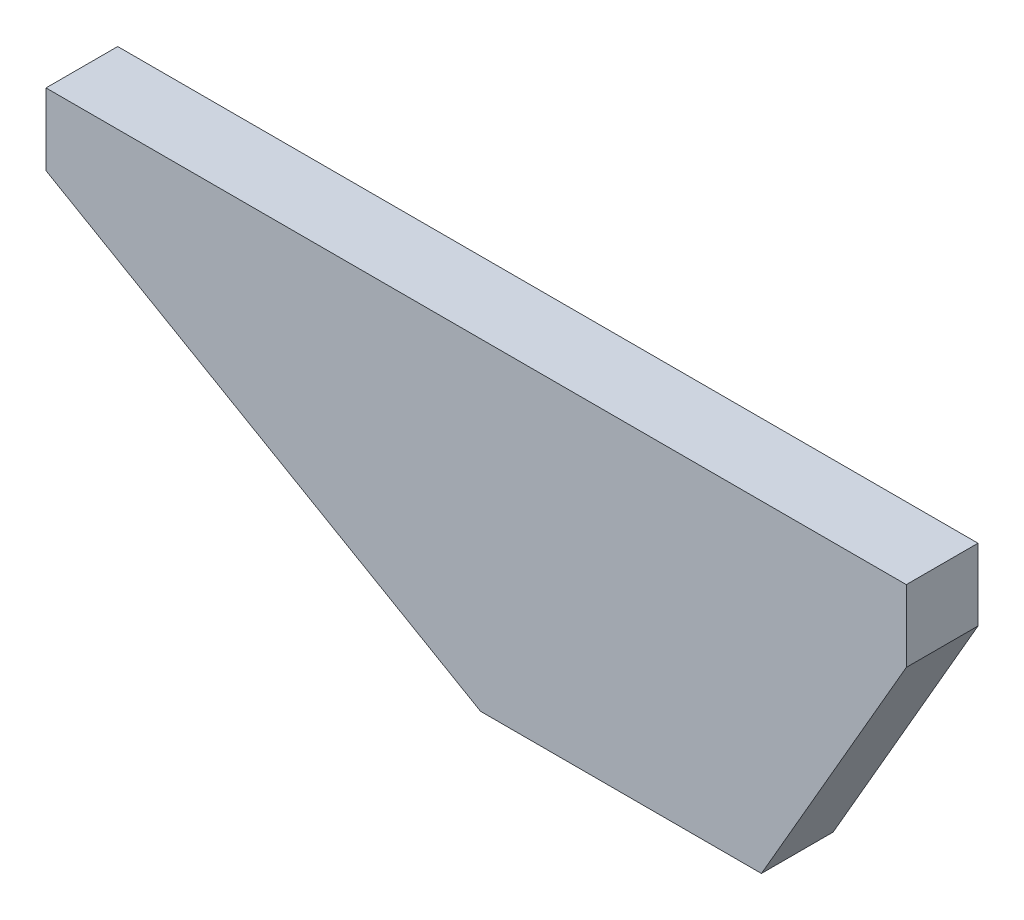
SolidWorks part; units mm, degrees
material "普通碳钢"
ref_plane "Front Plane" through (0, 0, 0) normal (0, 0, 1) x (1, 0, 0)
ref_plane "Top Plane" through (0, 0, 0) normal (0, 1, 0) x (1, 0, 0)
ref_plane "Right Plane" through (0, 0, 0) normal (1, 0, 0) x (0, 0, -1)
sketch "Sketch1" plane through (0, 0, 0) normal (0, 0, 1) x (1, 0, 0)
  line L0 (0, 0) -> (120, 0)
  line L2 (120, 0) -> (120, -10)
  line L3 (120, -10) -> (99.7927, -45)
  line L4 (99.7927, -45) -> (60.6218, -45)
  line L5 (60.6218, -45) -> (0, -10)
  line L6 (0, 0) -> (0, -10)
  dimension "D1" = 120
  dimension "D2" = 150
  dimension "D3" = 120
  dimension "D4" = 10
  dimension "D6" = 45
extrude "Boss-Extrude1" add sketch "Sketch1" along normal blind 10
